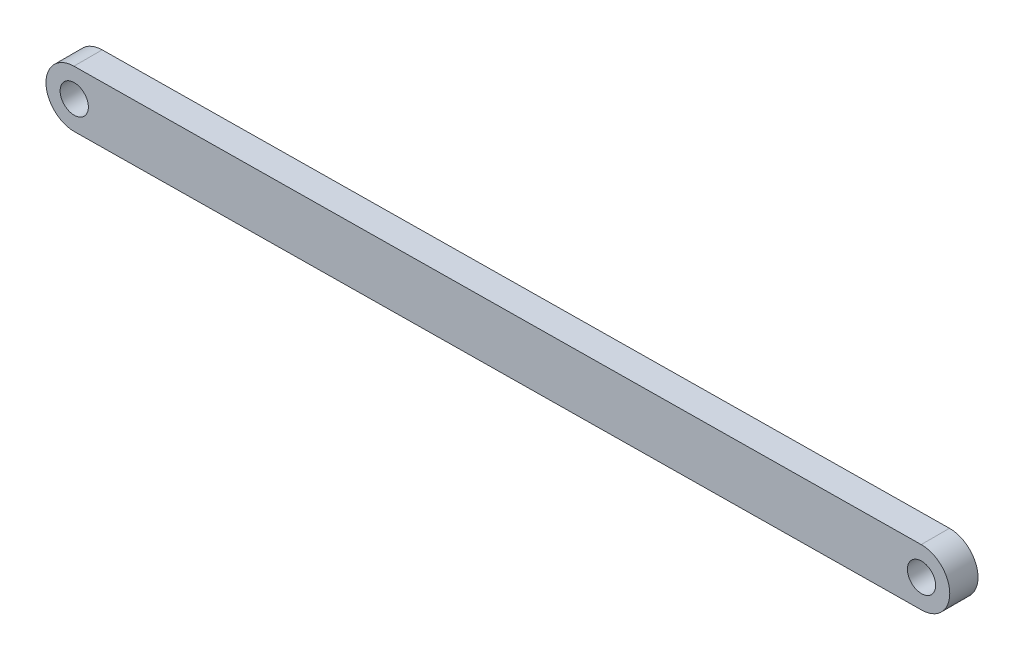
from build123d import *

# Parameters (mm, degrees)
SKETCH1_R           = 5
BOSS_EXTRUDE1_DEPTH = 10


with BuildPart() as part:
    # Sketch1 → Boss-Extrude1 (new body)
    with BuildSketch(Plane.XY):
        with BuildLine():
            Line((-0.109854152, 9.999396585), (299.8720434, 13.295021139))
            ThreePointArc((299.8720434, 13.295021139), (309.981294137, 3.405478706), (300.091751704, -6.703772031))
            Line((300.091751704, -6.703772031), (0.109854152, -9.999396585))
            ThreePointArc((0.109854152, -9.999396585), (-9.999396585, -0.109854152), (-0.109854152, 9.999396585))
        make_face()
        with Locations((299.981897552, 3.295624554)):
            Circle(SKETCH1_R, mode=Mode.SUBTRACT)
        Circle(SKETCH1_R, mode=Mode.SUBTRACT)
    extrude(amount=BOSS_EXTRUDE1_DEPTH)


solid = part.part
